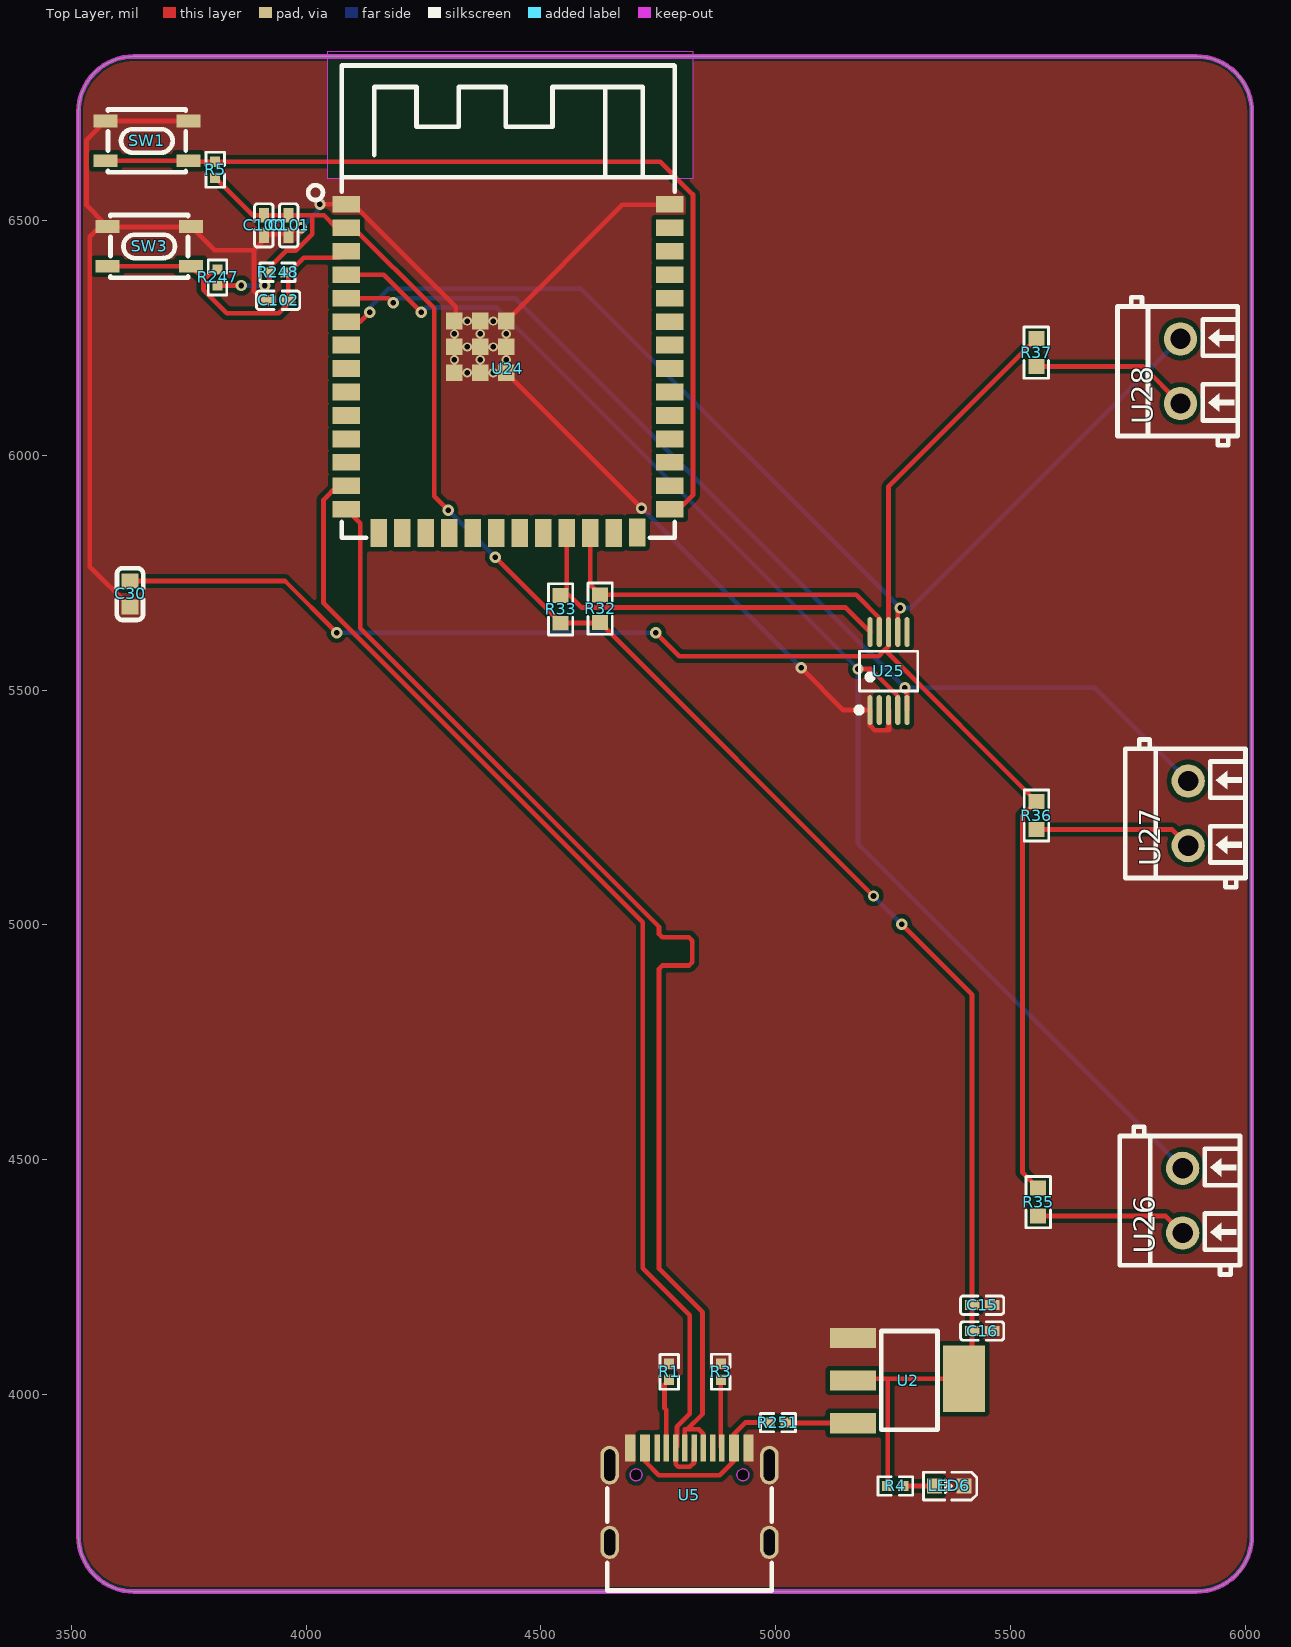
[diagram p0: Top Layer view]
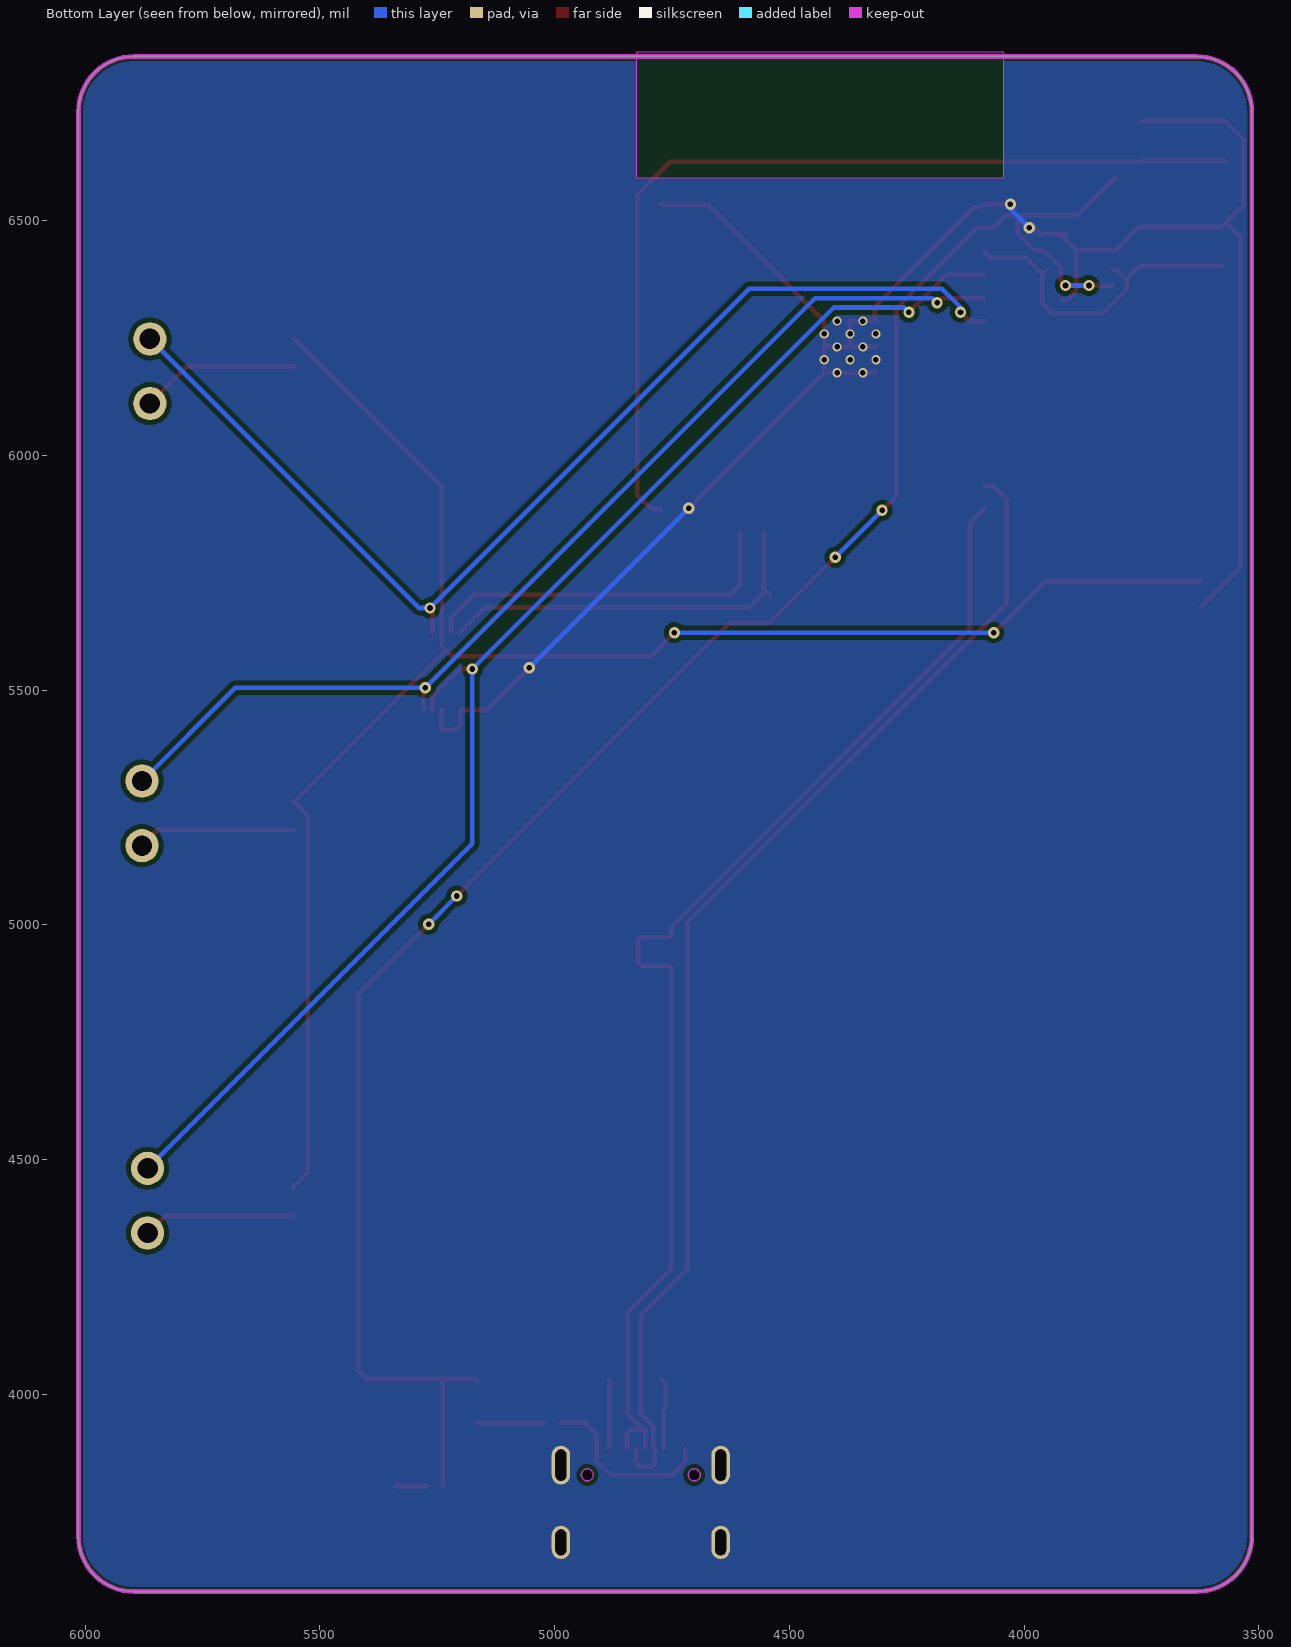
[diagram p1: Bottom Layer view, seen from below]
# Altium PCB MISC51586.pcbdoc
Units mil, origin at the board's own origin, x right, y up, seen from the top; angles counter-clockwise.
Board outline 2499.52 x 3270 mil, 2 copper layers (Top Layer, Bottom Layer), stack 62.206 mil thick; 28 components, 21 nets, 131 pads, 30 vias.

## Layer stack, top to bottom
Top Solder Mask Layer: solder mask 0.394, Dk 3.3
Top Layer: signal copper 1.379
Dielectric1: surface 59.449, FR4, Dk 4.5
Bottom Layer: signal copper 1.378
Bottom Solder Mask Layer: solder mask 0.394, Dk 3.3

## Board outline
3633.11,6850 ccw(c3633.11,6731.89) 3515,6731.89 3515,3698.11 ccw(c3633.11,3698.11) 3633.11,3580 5896.41,3580 ccw(c5896.41,3698.11) 6014.52,3698.11 6014.52,6731.89 ccw(c5896.41,6731.89) 5896.41,6850

## Design rules (kind name [scope] priority, off if disabled: settings)
BoardOutlineClearance copperThickness2oz_1 [All] p2 off: genericclearance=7.99 ignorepadtopadclearanceinfootprint=FALSE except(0: Arc-SplitContinuation Track-SplitContinuation SMDPad-SplitContinuation THPad-SplitContinuation Via-SplitContinuation Fill-SplitContinuation Region-SplitContinuation Poly-SplitContinuation Text-SplitContinuation Hole-SplitContinuation; 5.98: Arc-CutoutEdge Track-CutoutEdge SMDPad-CutoutEdge THPad-CutoutEdge Via-CutoutEdge Text-CutoutEdge; 6.89: Hole-OutlineEdge Hole-CutoutEdge; 10: Poly-OutlineEdge Poly-CutoutEdge; 11.81: Arc-OutlineEdge Track-OutlineEdge SMDPad-OutlineEdge THPad-OutlineEdge Via-OutlineEdge Fill-OutlineEdge Region-OutlineEdge Text-OutlineEdge Fill-CutoutEdge Region-CutoutEdge)
BoardOutlineClearance Plane_innerPlane_1 [All] p4 off: genericclearance=4.02 ignorepadtopadclearanceinfootprint=FALSE except(0: Arc-SplitContinuation Track-SplitContinuation SMDPad-SplitContinuation THPad-SplitContinuation Via-SplitContinuation Fill-SplitContinuation Region-SplitContinuation Poly-SplitContinuation Text-SplitContinuation Hole-SplitContinuation; 5.98: Arc-CutoutEdge Track-CutoutEdge SMDPad-CutoutEdge THPad-CutoutEdge Via-CutoutEdge Text-CutoutEdge; 6.89: Hole-OutlineEdge Hole-CutoutEdge; 10: Poly-OutlineEdge Poly-CutoutEdge; 11.81: Arc-OutlineEdge Track-OutlineEdge SMDPad-OutlineEdge THPad-OutlineEdge Via-OutlineEdge Fill-OutlineEdge Region-OutlineEdge Text-OutlineEdge Fill-CutoutEdge Region-CutoutEdge)
BoardOutlineClearance Copper_copperRegion_1 [All] p6 off: genericclearance=4.02 ignorepadtopadclearanceinfootprint=FALSE except(0: Arc-SplitContinuation Track-SplitContinuation SMDPad-SplitContinuation THPad-SplitContinuation Via-SplitContinuation Fill-SplitContinuation Region-SplitContinuation Poly-SplitContinuation Text-SplitContinuation Hole-SplitContinuation; 5.98: Arc-CutoutEdge Track-CutoutEdge SMDPad-CutoutEdge THPad-CutoutEdge Via-CutoutEdge Text-CutoutEdge; 6.89: Hole-OutlineEdge Hole-CutoutEdge; 10: Poly-OutlineEdge Poly-CutoutEdge; 11.81: Arc-OutlineEdge Track-OutlineEdge SMDPad-OutlineEdge THPad-OutlineEdge Via-OutlineEdge Fill-OutlineEdge Region-OutlineEdge Text-OutlineEdge Fill-CutoutEdge Region-CutoutEdge)
BoardOutlineClearance copperThickness1oz_1 [All] p8: genericclearance=4.02 ignorepadtopadclearanceinfootprint=FALSE except(0: Arc-SplitContinuation Track-SplitContinuation SMDPad-SplitContinuation THPad-SplitContinuation Via-SplitContinuation Fill-SplitContinuation Region-SplitContinuation Poly-SplitContinuation Text-SplitContinuation Hole-SplitContinuation; 5.98: Arc-CutoutEdge Track-CutoutEdge SMDPad-CutoutEdge THPad-CutoutEdge Via-CutoutEdge Text-CutoutEdge; 6.89: Hole-OutlineEdge Hole-CutoutEdge; 10: Poly-OutlineEdge Poly-CutoutEdge; 11.81: Arc-OutlineEdge Track-OutlineEdge SMDPad-OutlineEdge THPad-OutlineEdge Via-OutlineEdge Fill-OutlineEdge Region-OutlineEdge Text-OutlineEdge Fill-CutoutEdge Region-CutoutEdge)
Clearance copperThickness2oz [All] p1 off: gap=7.99 ignorepadtopadclearanceinfootprint=FALSE except(5.98: SMDPad-Track SMDPad-SMDPad THPad-Track SMDPad-THPad THPad-THPad Track-Via SMDPad-Via THPad-Via Via-Via Fill-SMDPad Region-SMDPad Fill-THPad Region-THPad Fill-Via Region-Via Fill-Fill Fill-Region Region-Region Arc-Track Arc-SMDPad Arc-THPad Arc-Via Fill-Arc Region-Arc Arc-Arc Text-Track SMDPad-Text Text-THPad Text-Via Fill-Text Region-Text Arc-Text Text-Text; 6.89: Hole-Track Hole-SMDPad Hole-THPad Hole-Via Fill-Hole Region-Hole Hole-Arc Hole-Text; 10: Poly-Track Poly-SMDPad Poly-THPad Poly-Via Poly-Fill Poly-Region Poly-Poly Poly-Arc Poly-Text Poly-Hole; 11.81: Fill-Track Region-Track)
Clearance Plane_innerPlane [All] p3 off: gap=4.02 ignorepadtopadclearanceinfootprint=FALSE except(5.98: SMDPad-Track SMDPad-SMDPad THPad-Track SMDPad-THPad THPad-THPad Track-Via SMDPad-Via THPad-Via Via-Via Fill-SMDPad Region-SMDPad Fill-THPad Region-THPad Fill-Via Region-Via Fill-Fill Fill-Region Region-Region Arc-Track Arc-SMDPad Arc-THPad Arc-Via Fill-Arc Region-Arc Arc-Arc Text-Track SMDPad-Text Text-THPad Text-Via Fill-Text Region-Text Arc-Text Text-Text; 6.89: Hole-Track Hole-SMDPad Hole-THPad Hole-Via Fill-Hole Region-Hole Hole-Arc Hole-Text; 10: Poly-Track Poly-SMDPad Poly-THPad Poly-Via Poly-Fill Poly-Region Poly-Poly Poly-Arc Poly-Text Poly-Hole; 11.81: Fill-Track Region-Track)
Clearance Copper_copperRegion [All] p5 off: gap=4.02 ignorepadtopadclearanceinfootprint=FALSE except(5.98: SMDPad-Track SMDPad-SMDPad THPad-Track SMDPad-THPad THPad-THPad Track-Via SMDPad-Via THPad-Via Via-Via Fill-SMDPad Region-SMDPad Fill-THPad Region-THPad Fill-Via Region-Via Fill-Fill Fill-Region Region-Region Arc-Track Arc-SMDPad Arc-THPad Arc-Via Fill-Arc Region-Arc Arc-Arc Text-Track SMDPad-Text Text-THPad Text-Via Fill-Text Region-Text Arc-Text Text-Text; 6.89: Hole-Track Hole-SMDPad Hole-THPad Hole-Via Fill-Hole Region-Hole Hole-Arc Hole-Text; 10: Poly-Track Poly-SMDPad Poly-THPad Poly-Via Poly-Fill Poly-Region Poly-Poly Poly-Arc Poly-Text Poly-Hole; 11.81: Fill-Track Region-Track)
Clearance copperThickness1oz [All] p7: gap=4.02 ignorepadtopadclearanceinfootprint=FALSE except(5.98: SMDPad-Track SMDPad-SMDPad THPad-Track SMDPad-THPad THPad-THPad Track-Via SMDPad-Via THPad-Via Via-Via Fill-SMDPad Region-SMDPad Fill-THPad Region-THPad Fill-Via Region-Via Fill-Fill Fill-Region Region-Region Arc-Track Arc-SMDPad Arc-THPad Arc-Via Fill-Arc Region-Arc Arc-Arc Text-Track SMDPad-Text Text-THPad Text-Via Fill-Text Region-Text Arc-Text Text-Text; 6.89: Hole-Track Hole-SMDPad Hole-THPad Hole-Via Fill-Hole Region-Hole Hole-Arc Hole-Text; 10: Poly-Track Poly-SMDPad Poly-THPad Poly-Via Poly-Fill Poly-Region Poly-Poly Poly-Arc Poly-Text Poly-Hole; 11.81: Fill-Track Region-Track)
DiffPairsRouting differentialPair [All] p1: maxlimit=6 minlimit=6 mostfreqgap=6 toplayer_minwidth=5 toplayer_prefwidth=10 toplayer_maxwidth=100 toplayer_mingap=6 toplayer_prefgap=6 toplayer_maxgap=6 bottomlayer_minwidth=5 bottomlayer_prefwidth=10 bottomlayer_maxwidth=100 bottomlayer_mingap=6 bottomlayer_prefgap=6 bottomlayer_maxgap=6 maxuncoupledlength=10
HoleToHoleClearance otherClearance [All] p1: gap=11.81 allowstackedmicrovias=TRUE
Length netLength [All] p1: minlimit=0 maxlimit=0
PasteMaskExpansion pasteMaskExpansion [All] p1: expansion=0
PlaneConnect innerPlane [All] p1: planeconnectstyle=Relief reliefexpansion=20 reliefentries=4 reliefconductorwidth=10 reliefairgap=10
PolygonConnect copperRegion [All] p1: connectstyle=Direct reliefconductorwidth=10 reliefentries=4 polygonreliefangle="90 Angle" airgapwidth=10 via.connectstyle=Relief via.reliefconductorwidth=10 via.reliefentries=4 via.polygonreliefangle="90 Angle" via.airgapwidth=10
RoutingVias viaSize [All] p1: holewidth=12.01 width=24.02 viastyle="Through Hole" minholewidth=11.81 minwidth=19.68 maxholewidth=248.03 maxwidth=393.7
SolderMaskExpansion solderMaskExpansion [IsVia] p1: expansion=-1000 istentingtop=TRUE
SolderMaskExpansion solderMaskExpansion [All] p2: expansion=2.01 istentingtop=FALSE
Width copperThickness2oz_2 [All] p1 off: maxlimit=100 minlimit=8 preferedwidth=10
Width copperThickness1oz_2 [All] p2: maxlimit=100 minlimit=5 preferedwidth=10

## Components (designator, comment, footprint, x,y, rotation, side; value= is the part's Value field where it differs from the comment)
C15 "100nF" C0402 5440,4190 r180 top
C16 "10uF" C0402 5440,4135 r180 top
C30 "100nF" C0603 3625,5705 r90 top
C100 "10uF" C0402 3910,6490 r90 top
C101 "100nF" C0402 3962.76,6490.05 r90 top
C102 "1uF" C0402 3940.35,6330.57 r0 top
LED6 "NCD0603R1" LED0603-RD_RED 5370,3805 r180 top
R1 "5.1K" r0402 4773.43,4048.06 r90 top
R3 "5.1K" r0402 4883.43,4048.17 r90 top
R4 "10K" r0402 5255,3805 r0 top
R5 "10K" r0402 3806.31,6608.63 r90 top
R32 "4.7K" R0603 4626.26,5673.55 r270 top
R33 "4.7K" R0603 4542.08,5672.31 r270 top
R35 "10K" R0603 5559.3,4409.64 r90 top
R36 "10K" R0603 5555.76,5233.02 r90 top
R37 "10K" R0603 5555.45,6219.2 r90 top
R247 "10K" r0402 3811.31,6379.1 r90 top
R248 "" r0402 3939.08,6390 r180 top
R251 "0" r0402 5005,3940 r0 top
SW1 "TS-1089S-02526" SW-SMD_4P-L4.2-W3.3-P2.15-LS5.1 3660.85,6670.03 r0 top
SW3 "TS-1089S-02526" SW-SMD_4P-L4.2-W3.3-P2.15-LS5.1 3665.85,6445.38 r0 top
U2 "AMS1117-3.3" sot-223(gd32) 5165,4120 r270 top
U5 "TYPE-C16P" USB-C-SMD_TYPE-C16PIN-SHOUHAN 4816.63,3785.21 r0 top
U24 "ESP32-S3-WROOM-1-N16R8" WIRELM-SMD_ESP32-S3-WROOM-1 4430,6185 r0 top
U25 "ADS1115IDGSR" MSOP-10_L3.0-W3.0-P0.50-LS5.0-BL 5240.63,5540.77 r0 top
U26 "DB301V-3.5-2P-GN-S" CONN-TH_DB301V-3.5-2P-GN 5867.16,4412.8 r90 top
U27 "DB301V-3.5-2P-GN-S" CONN-TH_DB301V-3.5-2P-GN 5878.93,5237.69 r90 top
U28 "DB301V-3.5-2P-GN-S" CONN-TH_DB301V-3.5-2P-GN 5862.37,6179.42 r90 top

## Footprints (in the part's own frame and the unit in brackets; to place one, negate y for a bottom-side part, rotate by r counter-clockwise, add the part's x,y. Pads: shape width x height; smd on the part's side, far side on the other; paste and mask are expansions set on the pad)
C0402 [mm]
  rect 0.79x0.54 smd paste-100 mask+0.051: 1(-0.545,0) 2(0.545,0)
  silkscreen extent -1.17,-0.5 1.17,0.5
C0603 [mm]
  rect 0.8x0.9 smd paste+0 mask+0.051: 1(-0.7,0) 2(0.7,0)
  silkscreen extent -1.41,-0.71 1.39,0.72
CONN-TH_DB301V-3.5-2P-GN [mm]
  round 1.8 hole 1.1: 1(-1.75,0) 2(1.75,0)
  silkscreen extent -4,-3.1 4,3.4
LED0603-RD_RED [mm]
  rect 0.8x0.8 smd: 1(-0.8,-0.003) 2(0.8,0.003)
  silkscreen extent -1.49,-0.75 1.39,0.76
MSOP-10_L3.0-W3.0-P0.50-LS5.0-BL [mm]
  oval 0.28x1.62 smd: 1(-1,-2.11) 2(-0.5,-2.11) 3(0,-2.11) 4(0.5,-2.11) 5(1,-2.11) 6(1,2.11) 7(0.5,2.11) 8(0,2.11) 9(-0.5,2.11) 10(-1,2.11)
  silkscreen extent -1.74,-2.26 1.58,1.07
r0402 [mm]
  rect 0.566x0.54 smd paste-100 mask+0.051: 1(-0.433,0) 2(0.433,0)
  silkscreen extent -0.94,-0.5 0.94,0.5
R0603 [mil]
  rect 31.75x34.02 smd paste-3937.01 mask+2: 1(-29.66,0) 2(29.66,0)
  silkscreen extent -55,-26 55,26
sot-223(gd32) [mm]
  rect 1.1x2.5 smd: 1(0,0) 2(2.3,0) 3(4.6,0)
  rect 3.6x2.29 smd: 4(2.2,6)
  silkscreen extent -0.38,1.52 4.95,4.57
SW-SMD_4P-L4.2-W3.3-P2.15-LS5.1 [mm]
  rect 1.3x0.7 smd: 1(-2.25,1.075) 2(2.25,1.075) 3(-2.25,-1.075) 4(2.25,-1.075)
  silkscreen extent -2.1,-1.7 2.1,1.7
USB-C-SMD_TYPE-C16PIN-SHOUHAN [mil]
  oval 39.4x82.7 hole 23.6 slot 66.9 at 90 deg paste+0 mask+2: 1(-170.1,64.2) 2(170.1,64.2)
  oval 39.4x70.9 hole 23.6 slot 55.1 at 90 deg paste+0 mask+2: 3(-170.1,-100.4) 4(170.1,-100.4)
  rect 21.7x57.1 smd paste-3937.01 mask+2: A1B12(-126,100.4) A4B9(-94.5,100.4) B1A12(126,100.4) B4A9(94.5,100.4)
  rect 11.8x57.1 smd paste-3937.01 mask+2: A5(-49.2,100.4) A6(-9.8,100.4) A7(9.8,100.4) A8(49.2,100.4) B5(68.9,100.4) B6(29.5,100.4) B7(-29.5,100.4) B8(-68.9,100.4)
  Board Outline Layer circle w0.1: c-113.8,43.3 r12.8
  Board Outline Layer circle w0.1: c113.8,43.3 r12.8
  Board Outline Layer region: -101,43.3 -102.27,37.75 -105.82,33.29 -110.95,30.82 -116.65,30.82 -121.78,33.29 -125.33,37.75 -126.6,43.3 -126.6,43.3 -125.33,48.85 -121.78,53.31 -116.65,55.78 -110.95,55.78 -105.82,53.31 -102.27,48.85 -101,43.3
  Board Outline Layer region: -101,43.3 -101.37,40.24 -102.47,37.35 -104.22,34.81 -106.53,32.77 -109.26,31.33 -112.26,30.59 -115.34,30.59 -118.34,31.33 -121.07,32.77 -123.38,34.81 -125.13,37.35 -126.23,40.24 -126.6,43.3 -126.23,46.36 -125.13,49.25 -123.38,51.79 -121.07,53.83 -118.34,55.27 -115.34,56.01 -112.26,56.01 -109.26,55.27 -106.53,53.83 -104.22,51.79 -102.47,49.25 -101.37,46.36
  Board Outline Layer region: 126.6,43.3 125.33,37.75 121.78,33.29 116.65,30.82 110.95,30.82 105.82,33.29 102.27,37.75 101,43.3 101,43.3 102.27,48.85 105.82,53.31 110.95,55.78 116.65,55.78 121.78,53.31 125.33,48.85 126.6,43.3
  Board Outline Layer region: 126.6,43.3 126.23,40.24 125.13,37.35 123.38,34.81 121.07,32.77 118.34,31.33 115.34,30.59 112.26,30.59 109.26,31.33 106.53,32.77 104.22,34.81 102.47,37.35 101.37,40.24 101,43.3 101.37,46.36 102.47,49.25 104.22,51.79 106.53,53.83 109.26,55.27 112.26,56.01 115.34,56.01 118.34,55.27 121.07,53.83 123.38,51.79 125.13,49.25 126.23,46.36
  Multi-Layer board cut-out: -101,43.3 -102.27,37.75 -105.82,33.29 -110.95,30.82 -116.65,30.82 -121.78,33.29 -125.33,37.75 -126.6,43.3 -126.6,43.3 -125.33,48.85 -121.78,53.31 -116.65,55.78 -110.95,55.78 -105.82,53.31 -102.27,48.85 -101,43.3
  Multi-Layer board cut-out: 126.6,43.3 125.33,37.75 121.78,33.29 116.65,30.82 110.95,30.82 105.82,33.29 102.27,37.75 101,43.3 101,43.3 102.27,48.85 105.82,53.31 110.95,55.78 116.65,55.78 121.78,53.31 125.33,48.85 126.6,43.3
  silkscreen extent -175,-203 175,14
WIRELM-SMD_ESP32-S3-WROOM-1 [mm]
  rect 1.5x0.9 smd paste+0 mask+0.05: 1(-8.75,8.895) 2(-8.75,7.625) 3(-8.75,6.355) 4(-8.75,5.085) 5(-8.75,3.815) 6(-8.75,2.545) 7(-8.75,1.275) 8(-8.75,0.005) 9(-8.75,-1.265) 10(-8.75,-2.535) 11(-8.75,-3.805) 12(-8.75,-5.075) 13(-8.75,-6.345) 14(-8.75,-7.615) 27(8.75,-7.615) 28(8.75,-6.345) 29(8.75,-5.075) 30(8.75,-3.805) 31(8.75,-2.535) 32(8.75,-1.265) 33(8.75,0.005) 34(8.75,1.275) 35(8.75,2.545) 36(8.75,3.815) 37(8.75,5.085) 38(8.75,6.355) 39(8.75,7.625) 40(8.75,8.895)
  rect 0.9x1.5 smd paste+0 mask+0.05: 15(-6.985,-8.895) 16(-5.715,-8.895) 17(-4.445,-8.895) 18(-3.175,-8.895) 19(-1.905,-8.895) 20(-0.635,-8.895) 21(0.635,-8.895) 22(1.905,-8.895) 23(3.175,-8.895) 24(4.445,-8.895) 25(5.715,-8.895) 26(6.985,-8.865)
  rect 0.9x0.9 smd: 41(-2.9,-0.225) 41(-2.9,1.175) 41(-2.9,2.575) 41(-1.5,-0.225) 41(-1.5,1.175) 41(-1.5,2.575) 41(-0.1,-0.225) 41(-0.1,1.175) 41(-0.1,2.575)
  silkscreen extent -10.81,-9.14 9.02,16.39

## Via types
v1: diameter 24.02, hole 12, Top Layer to Bottom Layer, 18 vias
v2: diameter 19.69, hole 11.8, Top Layer to Bottom Layer, 12 vias

## Nets (pads, with @x,y where several pads share a name; then routed paths per layer and width w, separated by ;. In a path a pad name is that pad's centre, name@x,y a point inside that pad or via, vN(x,y) a via of type N, cw(c..) or ccw(c..) an arc to the next point about the centre after c; other vN are vias at no path point)
5V: R251.2 U2.3 | length 143.4
  Top Layer w10: R251.2 5023.14,3938.9 U2.3
$1N1270: R1.1 U5.A5 | length 151.2
  Top Layer w10: U5.A5 4767.43,3967.02 4763.43,3971.02 4763.43,4021.02 R1.1
$1N1271: R3.1 U5.B5 | length 146.4
  Top Layer w10: R3.1 4883.43,3887.71 U5.B5
$1N1309: LED6.2 R4.2 | length 66.3
  Top Layer w10: R4.2@5272.18,3804.86 LED6.2
$1N12894: R35.1 U26.1 | length 322.8
  Top Layer w10: R35.1 5831.08,4379.98 U26.1
$1N12896: R36.1 U27.1 | length 337.5
  Top Layer w10: R36.1 5844.36,5203.36 U27.1
$1N12898: R37.1 U28.1 | length 339.7
  Top Layer w10: R37.1 5783.36,6189.54 U28.1
+3V3: C15.2 C16.2 C100.2 C101.2 R4.1 R5.1 R32.2 R33.2 R247.1 R248.2 U2.2 U2.4 U24.2 | length 4164.7
  Top Layer w10: R5.1 3886.39,6511.51 3910.05,6511.51 C101.2 4013.13,6511.51 ; R247.1 v1(3862.04,6362.06) ; v1(3912.04,6362.06) 3922.04,6372.06 R248.2 3922.42,6390.38 3922.42,6400.8 3957.78,6436.16 3977.78,6436.16 4013.13,6471.51 4013.13,6511.51 ; v1(4302.63,5883.2) 4272.63,5913.2 4272.63,6313.2 4100.63,6485.19 U24.2 4064.45,6485.19 4038.13,6511.51 4013.13,6511.51 ; v1(4402.63,5783.2) R33.2@4542.63,5643.2 ; R33.2 R33.2@4542.63,5643.2 ; R32.2 R32.2@4626.94,5643.2 ; U2.2 5168.94,4033.39 5238.72,4033.39 ; v1(5208.54,5061.61) R32.2@4626.94,5643.2 ; R4.1 5238.72,3805.76 5238.72,4033.39 ; v1(5268.54,5001.61) 5418.54,4851.61 C15.2 C16.2 5418.54,4050.71 U2.4 5238.72,4033.39 ; R33.2@4542.63,5643.2 R32.2@4626.94,5643.2
  Bottom Layer w10: v1(3862.04,6362.06) v1(3912.04,6362.06) ; v1(4302.63,5883.2) v1(4402.63,5783.2) ; v1(5208.54,5061.61) v1(5268.54,5001.61)
+5V: C30.2 R35.2 R36.2 R37.2 U25.8 | length 3783.4
  Top Layer w9.92: C30.2 3955,5732.56 v1(4065,5622.56) ; v1(4745,5622.56) 4795,5572.56 5219.34,5572.56 5231.62,5584.84 ; R37.2 5240.63,5934.03 U25.8 5240.63,5593.84 5231.62,5584.84 ; R36.2 5233.6,5584.84 5231.62,5584.84
  Top Layer w10: R36.2 5525.76,5232.68 5525.76,4472.84 R35.2
  Bottom Layer w9.92: v1(4065,5622.56) v1(4745,5622.56)
EN: C102.2 R247.2 R248.1 SW3.3 SW3.4 U24.3 | length 701.6
  Top Layer w10: SW3.3 SW3.4 3782.65,6374.84 3783.08,6374.84 ; R247.2 3804.38,6396.14 3783.08,6374.84 ; R248.1 R248.1@3960.04,6386.08 ; U24.3 4071.75,6421.44 3995.39,6421.44 R248.1@3960.04,6386.08 ; 3783.08,6374.84 3781.31,6373.07 3781.31,6353.07 3831.31,6303.07 3941.81,6303.07 3961.81,6323.07 C102.2 3961.81,6384.31 R248.1@3960.04,6386.08
GND: C15.1 C16.1 C30.1 C100.1 C101.1 C102.1 LED6.1 R1.2 R3.2 SW1.1 SW1.2 SW3.1 SW3.2 U2.1 U5.1 U5.2 U5.3 U5.4 U5.A1B12 U5.B1A12 U24.1 U24.40 U24.41 U25.1 U25.3 | length 4461.1
  Top Layer w9.92: U24.41@4426.06,6176.14 v1(4714.49,5887.7) ; v1(5054.49,5547.7) 5144.49,5457.7 U25.1 5201.26,5424.97 5211.46,5414.77 5241.46,5414.77 5241.46,5456.87 U25.3
  Top Layer w10: C30.1 3539.42,5763.02 3539.42,6465.56 SW3.1@3569.42,6495.56 ; SW1.2 SW1.1 3532.27,6672.35 3532.27,6532.71 SW3.1@3569.42,6495.56 ; SW3.2 SW3.2@3755.42,6486.72 ; C100.1 3912.51,6471.05 3922.72,6471.05 ; C102.1 3909.36,6330.57 3888.89,6351.05 3888.89,6437.22 ; C101.1 C101.1@3965.22,6471.05 ; v1(3989.36,6485.19) 3979.36,6485.19 C101.1@3965.22,6471.05 ; v1(4029.36,6535.19) U24.1 4092.2,6528.51 4106.31,6528.51 4318.44,6316.38 U24.41@4318.44,6286.38 ; U24.41@4315.82,6176.14 v2(4343.38,6176.14) 4370.94,6176.14 v2(4398.5,6176.14) 4426.06,6176.14 v2(4426.06,6203.7) U24.41@4426.06,6231.26 ; U24.41@4315.82,6231.26 v2(4343.38,6231.26) U24.41@4370.94,6231.26 ; U24.41@4315.82,6286.38 U24.41@4318.44,6286.38 ; U24.40 4773.16,6533.86 4673.55,6533.86 4426.06,6286.38 v2(4426.06,6258.81) U24.41@4426.06,6231.26 ; SW3.1@3569.42,6495.56 SW3.1 3578.26,6486.72 SW3.2@3755.42,6486.72 ; SW3.2@3755.42,6486.72 3804.92,6437.22 3888.89,6437.22 ; 3888.89,6437.22 3922.72,6471.05 ; 3922.72,6471.05 C101.1@3965.22,6471.05 ; U24.41@4318.44,6286.38 v2(4343.38,6286.37) 4370.94,6286.38 v2(4370.94,6258.81) U24.41@4370.94,6231.26 ; U24.41@4370.94,6231.26 v2(4398.5,6231.26) U24.41@4426.06,6231.26
  Bottom Layer w9.92: v1(4714.49,5887.7) v1(5054.49,5547.7)
  Bottom Layer w10: v1(3989.36,6485.19) 4029.36,6525.19 v1(4029.36,6535.19)
  other v2: 4315.82,6203.7 4370.94,6203.7 4315.82,6258.81 4398.5,6286.37
IO0: R5.2 SW1.3 SW1.4 U24.27 | length 1983.7
  Top Layer w10: SW1.3 SW1.4 3751.47,6625.67 R5.2 4754.02,6625.67 4824.02,6555.67 4824.02,5915.67 4793.54,5885.19 U24.27
SCL: R33.1 U24.23 U25.10 | length 824.2
  Top Layer w9.92: R33.1@4551.46,5711.36 4586.82,5676 5149.09,5676 U25.10
  Top Layer w10: R33.1 4551.46,5711.36 4555,5714.89 U24.23
SDA: R32.1 U24.24 U25.9 | length 785.5
  Top Layer w9.92: R32.1 5171.58,5703.21 5220.95,5653.84 U25.9
  Top Layer w10: U24.24 4605,5724.47 R32.1
STRESS-1: U24.4 U25.4 U26.2 | length 2934.8
  Top Layer w9.92: U24.4 4165.51,6385.19 v1(4245.51,6305.19) ; v1(5175.51,5545.19) 5202.82,5545.19 5260.32,5487.7 U25.4
  Bottom Layer w9.92: v1(4245.51,6305.19) 4255.51,6315.19 4405.51,6315.19 v1(5175.51,5545.19) 5175.51,5173.34 U26.2
STRESS-2: U24.5 U25.5 U27.2 | length 2277.1
  Top Layer w9.92: U24.5 4175.51,6335.19 v1(4185.51,6325.19) ; v1(5275.51,5505.19) 5280,5500.71 U25.5
  Bottom Layer w9.92: v1(4185.51,6325.19) 4195.51,6335.19 4445.51,6335.19 v1(5275.51,5505.19) 5680.32,5505.19 U27.2
STRESS-3: U24.6 U25.7 U28.2 | length 2384.3
  Top Layer w9.92: U24.6 4115.51,6285.19 v1(4135.51,6305.19) ; U25.7 5260.32,5670 v1(5265.51,5675.19)
  Bottom Layer w9.92: v1(4135.51,6305.19) 4135.51,6315.19 4175.51,6355.19 4585.51,6355.19 v1(5265.51,5675.19) 5289.25,5675.19 U28.2
STRESS-4: U25.6
USBD+: U5.A6 U5.B6 U24.14 | length 2526.4
  Top Layer w10: U24.14 4115.43,5855.27 4115.43,5632.01 4751.83,4995.61 4751.83,4980.66 4758.9,4973.59 4815.6,4973.59 4822.68,4966.52 4822.68,4920.66 4815.6,4913.59 4758.9,4913.59 4751.83,4906.52 4751.83,4267.84 4844.46,4175.2 4844.46,3958.25 4811.83,3925.61 ; U5.A6 4806.83,3925.61 4811.83,3925.61 ; U5.B6 4846.13,3916.31 4836.83,3925.61 4811.83,3925.61
USBD-: U5.A7 U5.B7 U24.13 | length 2526.5
  Top Layer w10: U24.13 4066.71,5935.19 4037.13,5905.61 4037.13,5685.61 4717.13,5005.61 4717.13,4268.66 4816.96,4168.83 4816.96,3958.35 4789.94,3931.33 4789.94,3888.43 U5.B7 4787.13,3851.38 4792.89,3845.61 4817.13,3845.61 4826.43,3854.91 U5.A7
VBUS: R251.1 U5.A4B9 U5.B4A9 | length 386.4
  Top Layer w10: U5.A4B9 4722.13,3857.11 4751.13,3828.11 4881.13,3828.11 4911.13,3858.11 U5.B4A9 4911.13,3915.61 4935.52,3940 R251.1
pads on no net: U5.A8 U5.B8 U24.7 U24.8 U24.9 U24.10 U24.11 U24.12 U24.15 U24.16 U24.17 U24.18 U24.19 U24.20 U24.21 U24.22 U24.25 U24.26 U24.28 U24.29 U24.30 U24.31 U24.32 U24.33 U24.34 U24.35 U24.36 U24.37 U24.38 U24.39 U25.2

## Polygon pours and split planes (outlines as drawn)
GND on Bottom Layer (solid, remove dead copper, pour order 2): 3350,6985 3350,3285 6700,3285 6700,6985
GND on Top Layer (solid, remove dead copper, pour order 0): 3000,7125 3000,3000 7085,3000 7085,7125

## Keep-outs
Board Outline Layer:
  region: 4045,6860 4045,6590 4825,6590 4825,6860
  lines w10: 3515,3698.11 3515,6731.89 cw(c3633.11,6731.89) 3633.11,6850 5896.41,6850 cw(c5896.41,6731.89) 6014.52,6731.89 6014.52,3698.11 cw(c5896.41,3698.11) 5896.41,3580 3633.11,3580 cw(c3633.11,3698.11) 3515,3698.11